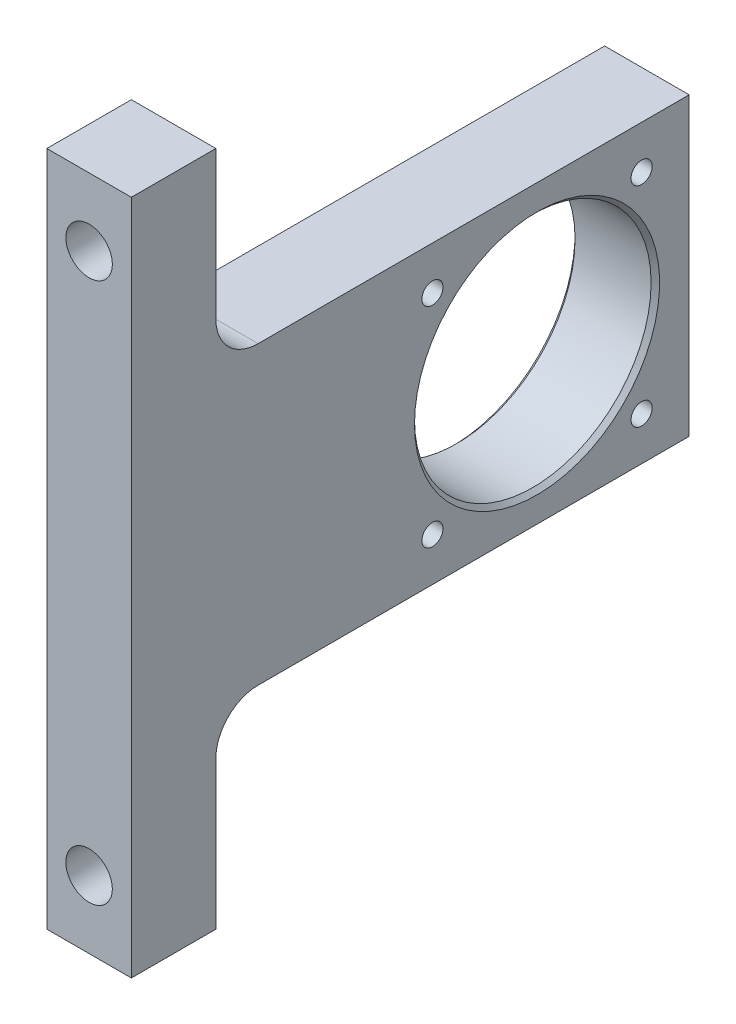
SolidWorks part; units mm, degrees
ref_plane "Front" through (0, 0, 0) normal (0, 0, 1) x (1, 0, 0)
ref_plane "Top" through (0, 0, 0) normal (0, 1, 0) x (1, 0, 0)
ref_plane "Right" through (0, 0, 0) normal (1, 0, 0) x (0, 0, -1)
sketch "Sketch1" plane through (0, 0, 0) normal (1, 0, 0) x (0, 0, -1)
  line L0 (0, -40) -> (0, 40)
  line L1 (0, 40) -> (10, 40)
  line L2 (10, 40) -> (10, 17.5)
  line L3 (10, 17.5) -> (66, 17.5)
  line L4 (66, 17.5) -> (66, -17.5)
  line L5 (66, -17.5) -> (10, -17.5)
  line L6 (10, -17.5) -> (10, -40)
  line L7 (10, -40) -> (0, -40)
  line L8 (0, 0) -> (66, 0) construction
  dimension "D1" = 66
  dimension "D2" = 10
  dimension "D3" = 35
  dimension "D4" = 80
extrude "Boss-Extrude1" add sketch "Sketch1" along normal blind 10
sketch "Sketch2" plane through (10, 0, 0) normal (1, 0, 0) x (0, 0, -1)
  line L0 (0, 40) -> (0, -40) construction
  circle A0 centre (48, 0) radius 14
  dimension "D2" = 28
  dimension "D1" = 48
extrude "Cut-Extrude1" cut sketch "Sketch2" against normal through all
hole_wizard "Ø5.5 (5.5) Diameter Hole1" positions "Sketch4" profile "Sketch3" hole size "Ø5.5" standard "ISO" end condition through all
sketch "Sketch4" plane through (0, 0, 0) normal (0, 0, 1) x (1, 0, 0)
  line L0 (0, 0) -> (10, 0) construction
  line L1 (0, 40) -> (0, -40) construction
  line L2 (10, 40) -> (10, -40) construction
  point P0 (5, 32)
  point P1 (5, -32)
  dimension "D1" = 64
  dimension "D2" = 5
sketch "Sketch3" plane through (5, 32, 0) normal (1, 0, 0) x (0, -1, 0)
  line L0 (0, 0) -> (0, 66)
  line L1 (0, 66) -> (2.75, 66)
  line L2 (2.75, 66) -> (2.75, 0)
  line L5 (2.75, 0) -> (0, 0)
  line L11 (0, -6.35) -> (0, 107.95) construction
  dimension "Thru Hole Dia." = 5.5
  dimension "Thru Hole Depth" = 66
hole_wizard "M3 Tapped Hole1" positions "Sketch6" profile "Sketch5" tap size "M3" standard "ISO" end condition through all
sketch "Sketch6" plane through (10, 0, 0) normal (1, 0, 0) x (0, 0, -1)
  line L2 (25.2033, 0) -> (70.4414, 0) construction
  line L5 (48, -21.3762) -> (48, 22.4423) construction
  line L8 (31.3971, -16.6029) -> (63.7196, 15.7196) construction
  line L11 (32.0526, 15.9474) -> (62.9527, -14.9527) construction
  circle A0 centre (48, 0) radius 17.5 construction
  point P0 (35.6256, 12.3744)
  point P1 (60.3744, 12.3744)
  point P3 (60.3744, -12.3744)
  point P5 (35.6256, -12.3744)
  dimension "D1" = 35
  dimension "D2" = 45
  dimension "D3" = 45
sketch "Sketch5" plane through (10, 12.3744, -35.6256) normal (0, 1, 0) x (0, 0, -1)
  line L0 (0, 0) -> (0, 10)
  line L1 (0, 10) -> (1.25, 10)
  line L2 (1.25, 10) -> (1.25, 0)
  line L5 (1.25, 0) -> (0, 0)
  line L11 (0, -6.35) -> (0, 107.95) construction
  dimension "Thru Tap Drill Dia." = 2.5
  dimension "Thru Tap Drill Depth" = 10
cosmetic thread "Hole Thread1" parameters "D2"=3
cosmetic thread "Hole Thread2" parameters "D2"=3
cosmetic thread "Hole Thread3" parameters "D2"=3
cosmetic thread "Hole Thread4" parameters "D2"=3
fillet "Fillet1" radius 5 2 edges at (5, 17.5, -10) (5, -17.5, -10)
chamfer "Chamfer1" distance 0.5 angle 45 2 edges at (0, 0, -62) (10, 0, -62)
